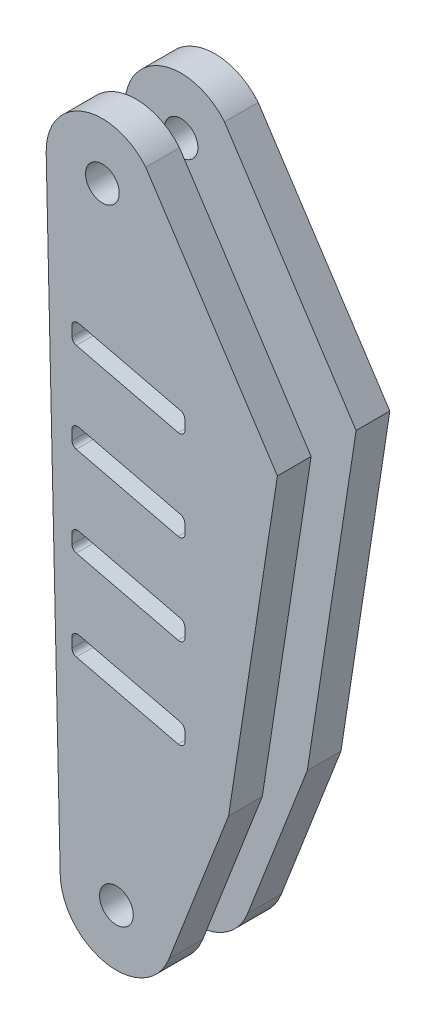
from build123d import *

# Parameters (mm, degrees)
SKETCH1_R               = 3
BOSS_EXTRUDE1_DEPTH     = 20
SKETCH2_W               = 70
SKETCH2_H               = 8
CUT_EXTRUDE1_DEPTH      = 60
CUT_EXTRUDE2_DEPTH      = 71
CUT_EXTRUDE2_DEPTH_BACK = 120
SKETCH3_W               = 44
SKETCH3_H               = 8
CUT_EXTRUDE3_START      = -60
SKETCH4_W               = 33.269827974
SKETCH4_H               = 8
CUT_EXTRUDE3_DEPTH      = 120
FILLET1_R               = 3
SKETCH5_W               = 12
SKETCH5_H               = 40
BOSS_EXTRUDE2_DEPTH     = 3
SCALE1_SCALE            = 0.5
CUT_EXTRUDE4_DEPTH      = 10
LPATTERN1_COUNT         = 40
LPATTERN1_PITCH         = 0.5
CUT_EXTRUDE6_DEPTH      = 10
FILLET3_R               = 0.5


with BuildPart() as part:
    # Sketch1 → Boss-Extrude1 (new body)
    with BuildSketch(Plane.XY):
        with BuildLine():
            Line((-76.796853281, 30.837882843), (-74.29959801, -79.133766728))
            ThreePointArc((-74.29959801, -79.133766728), (-66.029569813, -88.758525619), (-54.975215034, -82.527105996))
            Line((-54.975215034, -82.527105996), (-44.342640382, -55.142943195))
            Line((-44.342640382, -55.142943195), (-35.664684023, 1.573441942))
            Line((-35.664684023, 1.573441942), (-59.078548734, 37.420060128))
            ThreePointArc((-59.078548734, 37.420060128), (-70.281803918, 40.438970057), (-76.796853281, 30.837882843))
        make_face()
        with Locations((-66.79943059, 31.06490605)):
            Circle(SKETCH1_R, mode=Mode.SUBTRACT)
        with Locations((-64.29959801, -78.906684996)):
            Circle(SKETCH1_R, mode=Mode.SUBTRACT)
    extrude(amount=BOSS_EXTRUDE1_DEPTH)

    # Sketch2 → Cut-Extrude1 (cut)
    with BuildSketch(Plane(origin=(0, 0, 0), x_dir=(1, 0, 0), z_dir=(0, 1, 0))):
        with Locations((-76.79943059, -10)):
            Rectangle(SKETCH2_W, SKETCH2_H)
    extrude(amount=CUT_EXTRUDE1_DEPTH, mode=Mode.SUBTRACT)

    # Sketch3 → Cut-Extrude2 (cut, two sides: drawn at the far end of the back side and taken through both)
    with BuildSketch(Plane(origin=(0, 0, 0), x_dir=(1, 0, 0), z_dir=(0, 1, 0)).offset(-CUT_EXTRUDE2_DEPTH_BACK)):
        with Locations((-35.664684023, -10)):
            Rectangle(SKETCH3_W, SKETCH3_H)
    extrude(amount=CUT_EXTRUDE2_DEPTH + CUT_EXTRUDE2_DEPTH_BACK, mode=Mode.SUBTRACT)

    # Sketch4 → Cut-Extrude3 (cut)
    with BuildSketch(Plane(origin=(0, 0, 0), x_dir=(1, 0, 0), z_dir=(0, 1, 0)).offset(CUT_EXTRUDE3_START)):
        with Locations((-74.29959801, -10)):
            Rectangle(SKETCH4_W, SKETCH4_H)
    extrude(amount=-CUT_EXTRUDE3_DEPTH, mode=Mode.SUBTRACT)

    # Fillet1
    fillet1_edges = [part.edges().sort_by_distance(p)[0] for p in [
        (-76.096581295, 0, 10),
        (-57.664684023, 0, 10),
        (-57.664684023, -60, 10),
        (-74.7340909, -60, 10),
    ]]
    fillet(fillet1_edges, radius=FILLET1_R)

    # Sketch5 → Boss-Extrude2 (add)
    with BuildSketch(Plane(origin=(-76.05736147, -1.727123741, 0), x_dir=(0, 0, 1), z_dir=(-0.9997422691059525, -0.022702320649687743, 0))):
        with Locations((10, -27.839999236)):
            Rectangle(SKETCH5_W, SKETCH5_H)
    extrude(amount=BOSS_EXTRUDE2_DEPTH)


with BuildPart() as part_1:
    # Scale1: scaled about (0, 0, 0)
    add(part.part.scale(SCALE1_SCALE))

    # Sketch6 → Cut-Extrude4 (cut)
    with BuildSketch(Plane.XY.offset(8)):
        Polygon((-39.43930105, -4.816604664), (-39.183624007, -5.072281708), (-39.427946964, -5.316604664), align=None)
    cut_extrude4 = extrude(amount=-CUT_EXTRUDE4_DEPTH, mode=Mode.SUBTRACT)

    # LPattern1: Cut-Extrude4 ×40
    with Locations(*[Vector(0.02270232064968673, -0.9997422691059525, 0) * (i * LPATTERN1_PITCH) for i in range(1, LPATTERN1_COUNT)]):
        add(cut_extrude4, mode=Mode.SUBTRACT)

    # Sketch7 → Cut-Extrude6 (cut)
    with BuildSketch(Plane.XY.offset(10)):
        Polygon((-26.077673432, 1.430161372), (-36.135224219, 3.850999592), (-36.092915521, 1.98785116), (-26.035364734, -0.43298706), align=None)
        Polygon((-26.077673432, -6.569838628), (-36.135224219, -4.149000408), (-36.092915521, -6.01214884), (-26.035364734, -8.43298706), align=None)
        Polygon((-26.077673432, -14.569838628), (-36.135224219, -12.149000408), (-36.092915521, -14.01214884), (-26.035364734, -16.43298706), align=None)
        Polygon((-26.077673432, -22.569838628), (-36.135224219, -20.149000408), (-36.092915521, -22.01214884), (-26.035364734, -24.43298706), align=None)
    extrude(amount=-CUT_EXTRUDE6_DEPTH, mode=Mode.SUBTRACT)

    # Fillet3
    fillet3_edges = [part_1.edges().sort_by_distance(p)[0] for p in [
        (-26.077673432, 1.430161372, 1.5),
        (-26.035364734, -0.43298706, 1.5),
        (-36.092915521, 1.98785116, 1.5),
        (-36.135224219, 3.850999592, 1.5),
        (-26.077673432, 1.430161372, 8.5),
        (-26.035364734, -0.43298706, 8.5),
        (-36.092915521, 1.98785116, 8.5),
        (-36.135224219, 3.850999592, 8.5),
        (-26.077673432, -6.569838628, 1.5),
        (-28.832342012, -7.759758594, 5),
        (-28.832342012, -5.906793805, 5),
        (-26.077673432, -6.569838628, 8.5),
        (-26.035364734, -8.43298706, 8.5),
        (-26.035364734, -8.43298706, 1.5),
        (-36.092915521, -6.01214884, 5),
        (-36.135224219, -4.149000408, 5),
        (-26.077673432, -14.569838628, 1.5),
        (-28.832342012, -15.759758594, 5),
        (-28.832342012, -13.906793805, 5),
        (-26.077673432, -14.569838628, 8.5),
        (-26.035364734, -16.43298706, 8.5),
        (-26.035364734, -16.43298706, 1.5),
        (-36.092915521, -14.01214884, 5),
        (-36.135224219, -12.149000408, 5),
        (-26.077673432, -22.569838628, 1.5),
        (-28.832342012, -23.759758594, 5),
        (-28.832342012, -21.906793805, 5),
        (-26.077673432, -22.569838628, 8.5),
        (-26.035364734, -24.43298706, 8.5),
        (-26.035364734, -24.43298706, 1.5),
        (-36.092915521, -22.01214884, 5),
        (-36.135224219, -20.149000408, 5),
    ]]
    fillet(fillet3_edges, radius=FILLET3_R)


solid = part_1.part
